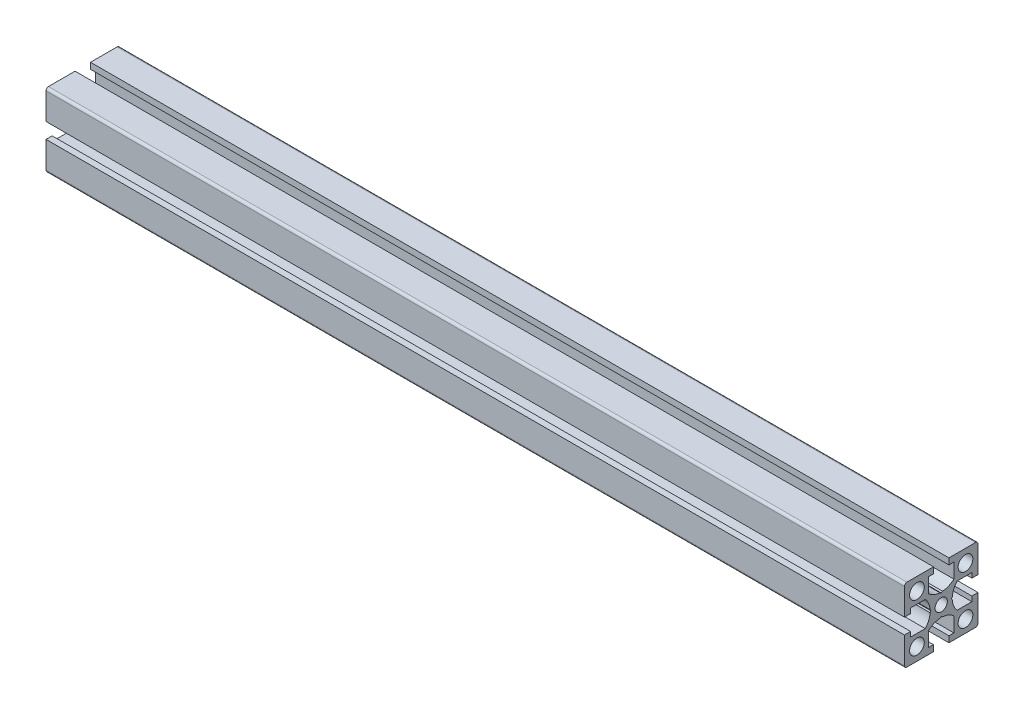
SolidWorks part; units mm, degrees
ref_plane "前视基准面" through (0, 0, 0) normal (0, 0, 1) x (1, 0, 0)
ref_plane "上视基准面" through (0, 0, 0) normal (0, 1, 0) x (1, 0, 0)
ref_plane "右视基准面" through (0, 0, 0) normal (1, 0, 0) x (0, 0, -1)
sketch "草图1" plane through (0, 0, 0) normal (0, 0, 1) x (1, 0, 0)
  line L0 (0, 0) -> (350, 0)
  line L1 (16.5, 0) -> (-16.5, 0) construction
  dimension "D1" = 350
other "0国耀铝型材 GY-3030国标铝型材(1)"
ref_plane "基准面1" through (0, 0, 0) normal (1, 0, 0) x (0, 1, 0)
sketch "草图11" plane through (0, 0, 0) normal (1, 0, 0) x (0, 1, 0)
  line L0 (0, 0) -> (15, 0) construction
  line L1 (0, 0) -> (0, 15) construction
  line L42 (-14, -15) -> (-3.15, -15)
  line L43 (-3.15, -15) -> (-3.15, -12.5)
  line L44 (-3.15, -12.5) -> (-5.15, -12.5)
  line L45 (-5.15, -12.5) -> (-5.15, -6.5)
  line L46 (-0.555, -4.52) -> (0, -4.2)
  line L47 (0, -4.2) -> (0.555, -4.52)
  line L48 (5.15, -6.5) -> (5.15, -12.5)
  line L49 (5.15, -12.5) -> (3.15, -12.5)
  line L50 (3.15, -12.5) -> (3.15, -15)
  line L51 (3.15, -15) -> (14, -15)
  line L52 (15, -14) -> (15, -3.15)
  line L53 (15, -3.15) -> (12.5, -3.15)
  line L54 (12.5, -3.15) -> (12.5, -5.15)
  line L55 (12.5, -5.15) -> (6.5, -5.15)
  line L56 (4.52, -0.554) -> (4.2, 0)
  line L57 (4.2, 0) -> (4.52, 0.555)
  line L58 (6.5, 5.15) -> (12.5, 5.15)
  line L59 (12.5, 5.15) -> (12.5, 3.15)
  line L60 (12.5, 3.15) -> (15, 3.15)
  line L61 (15, 3.15) -> (15, 14)
  line L62 (14, 15) -> (3.15, 15)
  line L63 (3.15, 15) -> (3.15, 12.5)
  line L64 (3.15, 12.5) -> (5.15, 12.5)
  line L65 (5.15, 12.5) -> (5.15, 6.5)
  line L66 (0.555, 4.521) -> (0, 4.2)
  line L67 (0, 4.2) -> (-0.555, 4.521)
  line L68 (-5.15, 6.5) -> (-5.15, 12.5)
  line L69 (-5.15, 12.5) -> (-3.15, 12.5)
  line L70 (-3.15, 12.5) -> (-3.15, 15)
  line L71 (-3.15, 15) -> (-14, 15)
  line L72 (-15, 14) -> (-15, 3.15)
  line L73 (-15, 3.15) -> (-12.5, 3.15)
  line L74 (-12.5, 3.15) -> (-12.5, 5.15)
  line L75 (-12.5, 5.15) -> (-6.5, 5.15)
  line L76 (-4.52, 0.555) -> (-4.2, 0)
  line L77 (-4.2, 0) -> (-4.52, -0.554)
  line L78 (-6.5, -5.15) -> (-12.5, -5.15)
  line L79 (-12.5, -5.15) -> (-12.5, -3.15)
  line L80 (-12.5, -3.15) -> (-15, -3.15)
  line L81 (-15, -3.15) -> (-15, -14)
  arc A13 (-15, -14) -> (-14, -15) centre (-14, -14) ccw
  arc A14 (-5.15, -6.5) -> (-0.555, -4.52) centre (0.0004, -12.1308) cw
  arc A15 (0.555, -4.52) -> (5.15, -6.5) centre (-0.0004, -12.1308) cw
  arc A16 (14, -15) -> (15, -14) centre (14, -14) ccw
  arc A17 (6.5, -5.15) -> (4.52, -0.554) centre (12.1308, 0.0003) cw
  arc A18 (4.52, 0.555) -> (6.5, 5.15) centre (12.1308, -0.0004) cw
  arc A19 (15, 14) -> (14, 15) centre (14, 14) ccw
  arc A20 (5.15, 6.5) -> (0.555, 4.521) centre (0.0008, 12.1318) cw
  arc A21 (-0.555, 4.521) -> (-5.15, 6.5) centre (-0.0008, 12.1318) cw
  arc A22 (-14, 15) -> (-15, 14) centre (-14, 14) ccw
  arc A23 (-6.5, 5.15) -> (-4.52, 0.555) centre (-12.1308, -0.0004) cw
  arc A24 (-4.52, -0.554) -> (-6.5, -5.15) centre (-12.1308, 0.0003) cw
  circle A25 centre (9.8, 9.9) radius 3
  circle A26 centre (9.8, -9.9) radius 3
  circle A27 centre (0, 0) radius 2.5
  circle A28 centre (-9.8, 9.9) radius 3
  circle A29 centre (-10, -9.9) radius 3
  point P0 (0, 0)
  dimension "D3" = 19.8
  dimension "D2" = 19.8
  dimension "D5" = 5
  dimension "D6" = 6
  dimension "D4" = 6.3
  dimension "D9" = 30
  dimension "D10" = 30
